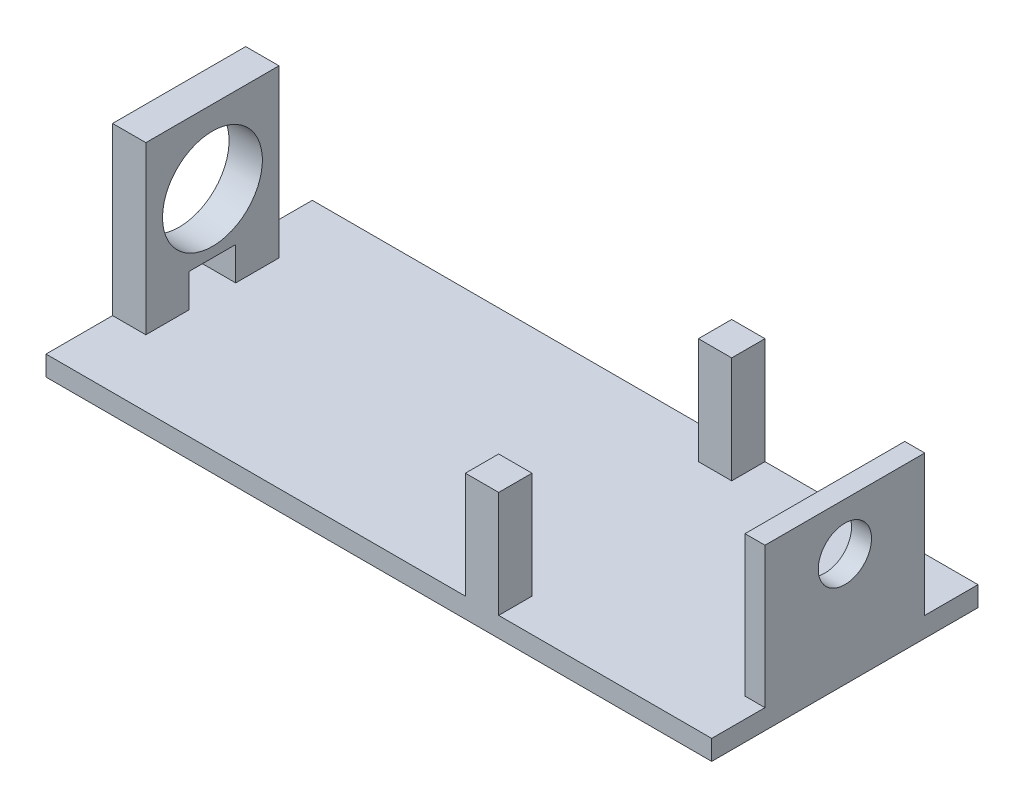
from build123d import *

# Parameters (mm, degrees)
SKETCH1_W           = 100
SKETCH1_H           = 40
BOSS_EXTRUDE1_DEPTH = 3
SKETCH2_W           = 20
SKETCH2_H           = 25
SKETCH2_R           = 7.5
BOSS_EXTRUDE2_DEPTH = 5
SKETCH3_R           = 7.5
BOSS_EXTRUDE3_DEPTH = 5
SKETCH4_W           = 5
SKETCH4_H           = 16
BOSS_EXTRUDE4_DEPTH = 5
SKETCH7_W           = 24
SKETCH7_H           = 24.131684527
SKETCH7_R           = 4
BOSS_EXTRUDE5_DEPTH = 3
SKETCH9_W           = 8.913505449
SKETCH9_H           = 22.920442584
CUT_EXTRUDE3_DEPTH  = 47


with BuildPart() as part:
    # Sketch1 → Boss-Extrude1 (new body)
    with BuildSketch(Plane(origin=(0, 0, 0), x_dir=(1, 0, 0), z_dir=(0, 1, 0))):
        Rectangle(SKETCH1_W, SKETCH1_H)
    extrude(amount=BOSS_EXTRUDE1_DEPTH)

    # Sketch2 → Boss-Extrude2 (add)
    with BuildSketch(Plane(origin=(40, 0, 0), x_dir=(0, 0, -1), z_dir=(1, 0, 0))):
        with Locations((0, 15.5)):
            Rectangle(SKETCH2_W, SKETCH2_H)
        with Locations((0, 17)):
            Circle(SKETCH2_R, mode=Mode.SUBTRACT)
    extrude(amount=BOSS_EXTRUDE2_DEPTH)

    # Sketch3 → Boss-Extrude3 (add)
    with BuildSketch(Plane.ZY.offset(50)):
        Polygon((-10, 3), (-3.5, 3), (-3.5, 8), (3.5, 8), (3.5, 3), (10, 3), (10, 28), (-10, 28), align=None)
        with Locations(Location((0, 17, 0), (0, 0, 180))):
            Circle(SKETCH3_R, mode=Mode.SUBTRACT)
    extrude(amount=-BOSS_EXTRUDE3_DEPTH)

    # Sketch4 → Boss-Extrude4 (add)
    with BuildSketch(Plane(origin=(13, 0, 0), x_dir=(0, 0, -1), z_dir=(1, 0, 0))):
        with Locations((17.5, 11)):
            Rectangle(SKETCH4_W, SKETCH4_H)
        with Locations((-17.5, 11)):
            Rectangle(SKETCH4_W, SKETCH4_H)
    extrude(amount=BOSS_EXTRUDE4_DEPTH)

    # Sketch7 → Boss-Extrude5 (add)
    with BuildSketch(Plane(origin=(50, 0, 0), x_dir=(0, 0, -1), z_dir=(1, 0, 0))):
        with Locations((0, 12.065842264)):
            Rectangle(SKETCH7_W, SKETCH7_H)
        with Locations((0, 17)):
            Circle(SKETCH7_R, mode=Mode.SUBTRACT)
    extrude(amount=-BOSS_EXTRUDE5_DEPTH)

    # Sketch9 → Cut-Extrude3 (cut)
    with BuildSketch(Plane(origin=(0, 3, 0), x_dir=(1, 0, 0), z_dir=(0, 1, 0))):
        with Locations((40.747453483, 0)):
            Rectangle(SKETCH9_W, SKETCH9_H)
    extrude(amount=CUT_EXTRUDE3_DEPTH, mode=Mode.SUBTRACT)


solid = part.part
